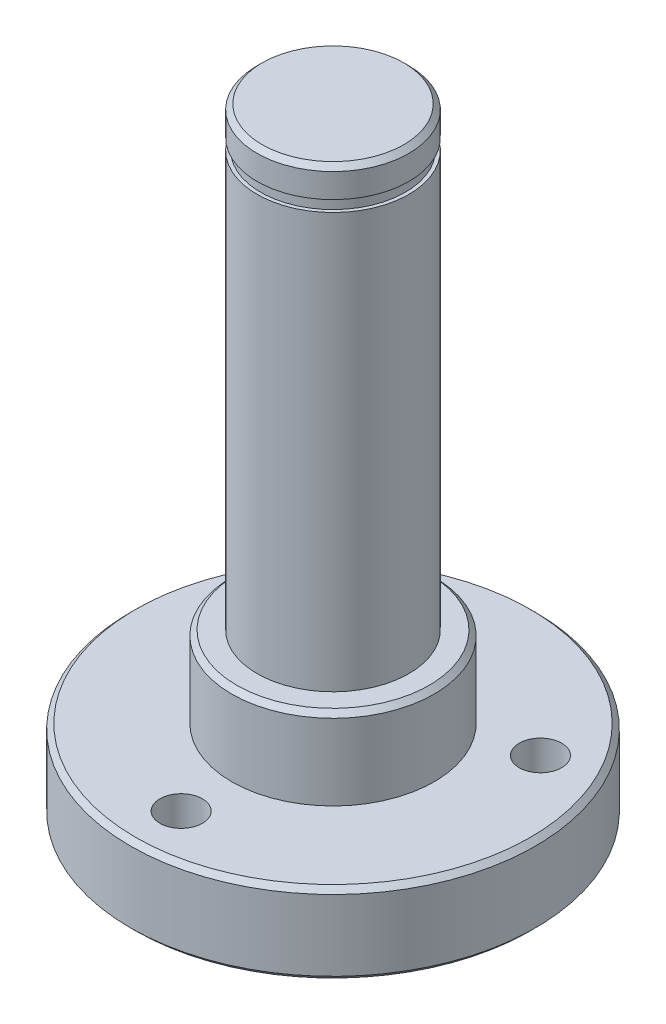
from build123d import *

# Parameters (mm, degrees)
SKETCH_1_R         = 20
EXTRUDE_1_DEPTH    = 4
SKETCH_2_R         = 10
EXTRUDE_2_DEPTH    = 8
SKETCH_3_R         = 7.5
EXTRUDE_3_DEPTH    = 45
SKETCH_4_W         = 0.35
SKETCH_4_H         = 1.1
HOLE_WIZARD_M5_1_D = 4.2
CHAMFER_1_SIZE     = 0.5
CHAMFER_2_SIZE     = 0.5


with BuildPart() as part:
    # 草图1 → 凸台-拉伸1 (new, symmetric)
    with BuildSketch(Plane(origin=(0, 0, 0), x_dir=(1, 0, 0), z_dir=(0, 1, 0))):
        with Locations(Location((0, 0, 0), (0, 0, 270))):
            Circle(SKETCH_1_R)
    extrude(amount=EXTRUDE_1_DEPTH, both=True)

    # 草图2 → 凸台-拉伸2 (add)
    with BuildSketch(Plane(origin=(0, 4, 0), x_dir=(1, 0, 0), z_dir=(0, 1, 0))):
        with Locations(Location((0, 0, 0), (0, 0, 270))):
            Circle(SKETCH_2_R)
    extrude(amount=EXTRUDE_2_DEPTH)

    # 草图3 → 凸台-拉伸3 (add)
    with BuildSketch(Plane(origin=(0, 12, 0), x_dir=(1, 0, 0), z_dir=(0, 1, 0))):
        with Locations(Location((0, 0, 0), (0, 0, 90))):
            Circle(SKETCH_3_R)
    extrude(amount=EXTRUDE_3_DEPTH)

    # 草图4 → 切除-旋转1 (revolve, cut)
    with BuildSketch(Plane(origin=(0, 0, 0), x_dir=(0, 0, -1), z_dir=(1, 0, 0))):
        with Locations((7.325, 53.55)):
            Rectangle(SKETCH_4_W, SKETCH_4_H)
    revolve(axis=Axis((0, 0, 0), (0, 1, 0)), mode=Mode.SUBTRACT)

    # M5 螺纹孔1 (through all)
    with Locations(Plane(origin=(0, 4, 0), x_dir=(1, 0, 0), z_dir=(0, 1, 0))):
        with Locations((-12.990381057, 7.5), (12.990381057, 7.5), (0, -15)):
            Hole(HOLE_WIZARD_M5_1_D / 2)

    # 倒角1
    chamfer_1_edges = [part.edges().sort_by_distance(p)[0] for p in [
        (0, 57, 7.5),
        (0, 12, -10),
    ]]
    chamfer(chamfer_1_edges, length=CHAMFER_1_SIZE)

    # 倒角2
    chamfer_2_edges = [part.edges().sort_by_distance(p)[0] for p in [
        (0, -4, -20),
        (0, 4, -20),
    ]]
    chamfer(chamfer_2_edges, length=CHAMFER_2_SIZE)


solid = part.part
